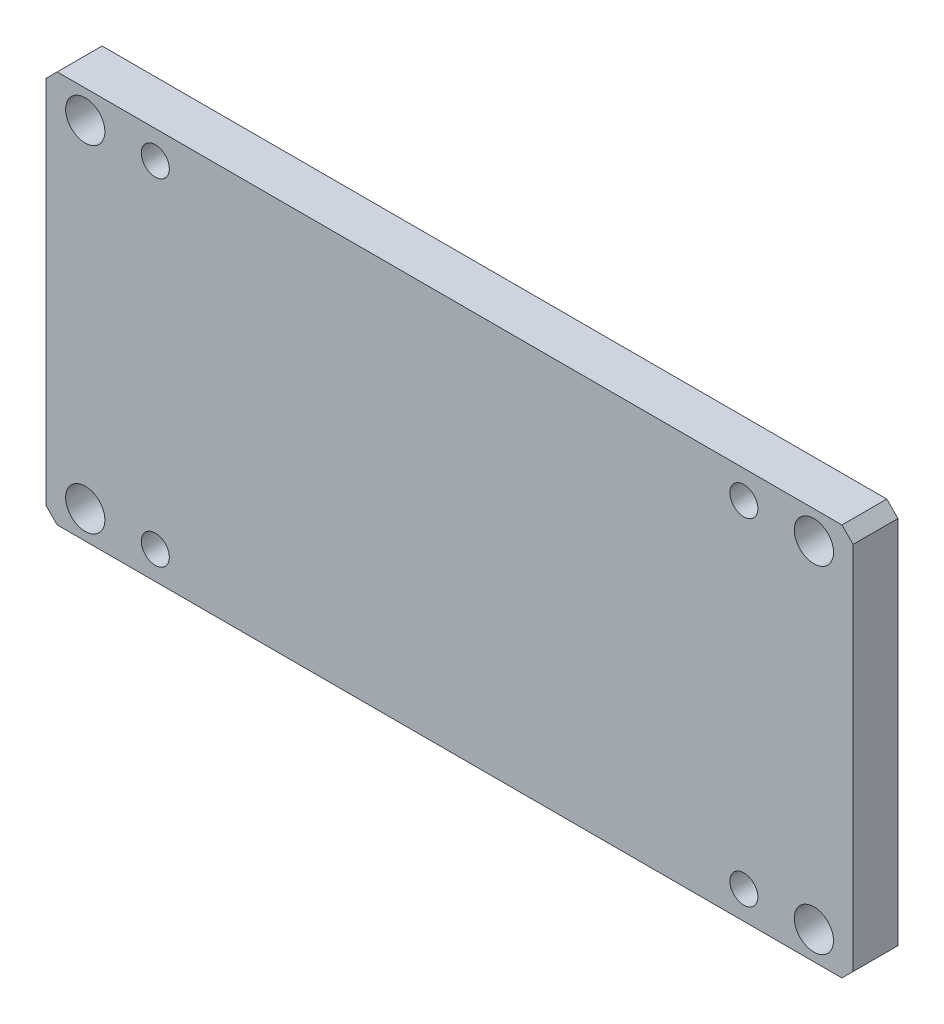
from build123d import *

# Parameters (mm, degrees)
SKETCH1_W           = 144
SKETCH1_H           = 70
SKETCH1_R           = 3.5
BOSS_EXTRUDE1_DEPTH = 8
CHAMFER1_SIZE       = 2
M6_TAPPED_HOLE1_D   = 5


with BuildPart() as part:
    # Sketch1 → Boss-Extrude1 (new body)
    with BuildSketch(Plane.XY):
        Rectangle(SKETCH1_W, SKETCH1_H)
        with Locations((65, 30)):
            Circle(SKETCH1_R, mode=Mode.SUBTRACT)
        with Locations((65, -30)):
            Circle(SKETCH1_R, mode=Mode.SUBTRACT)
        with Locations((-65, -30)):
            Circle(SKETCH1_R, mode=Mode.SUBTRACT)
        with Locations((-65, 30)):
            Circle(SKETCH1_R, mode=Mode.SUBTRACT)
    extrude(amount=BOSS_EXTRUDE1_DEPTH)

    # Chamfer1
    chamfer1_edges = [part.edges().sort_by_distance(p)[0] for p in [
        (-72, -35, 4),
        (-72, 35, 4),
        (72, 35, 4),
        (72, -35, 4),
    ]]
    chamfer(chamfer1_edges, length=CHAMFER1_SIZE)

    # M6 Tapped Hole1 (through all)
    with Locations(Plane.XY.offset(8)):
        with Locations((-52.5, 30), (-52.5, -30), (52.5, -30), (52.5, 30)):
            Hole(M6_TAPPED_HOLE1_D / 2)


solid = part.part
